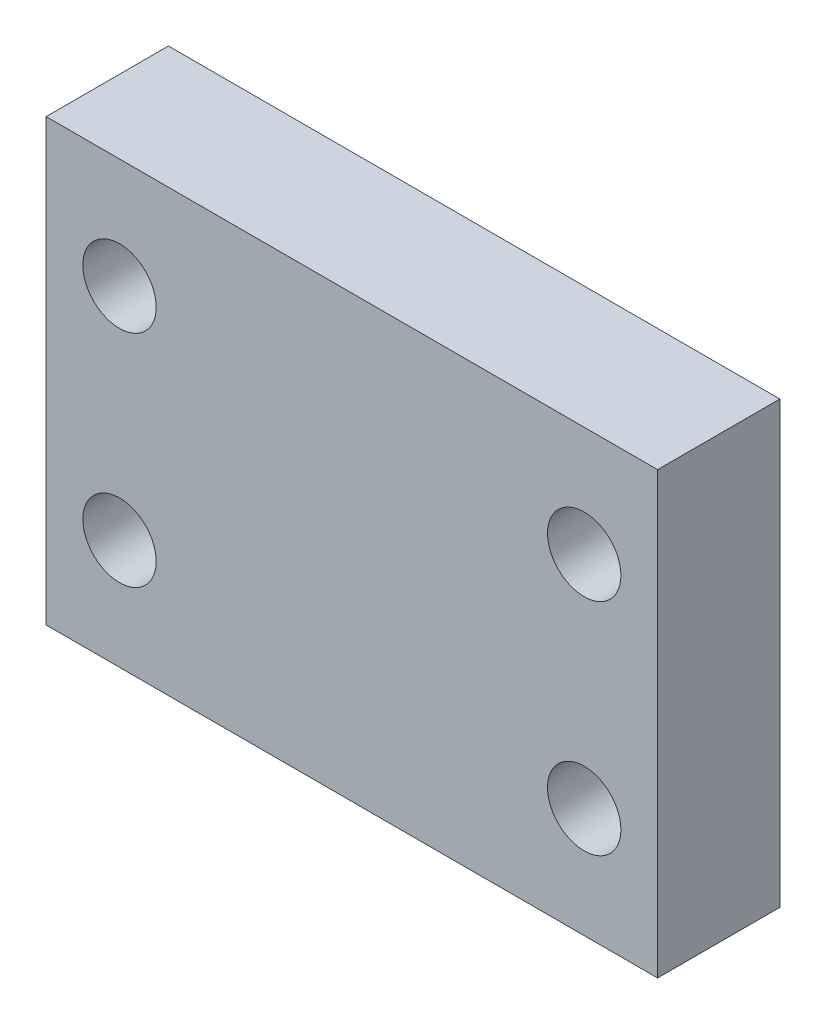
from build123d import *

# Parameters (mm, degrees)
SKETCH1_W           = 25
SKETCH1_H           = 18
SKETCH1_R           = 1.5
BOSS_EXTRUDE1_DEPTH = 5


with BuildPart() as part:
    # Sketch1 → Boss-Extrude1 (new body)
    with BuildSketch(Plane.XY):
        Rectangle(SKETCH1_W, SKETCH1_H)
        with Locations((-9.5, 4.5)):
            Circle(SKETCH1_R, mode=Mode.SUBTRACT)
        with Locations((9.5, 4.5)):
            Circle(SKETCH1_R, mode=Mode.SUBTRACT)
        with Locations((9.5, -4.5)):
            Circle(SKETCH1_R, mode=Mode.SUBTRACT)
        with Locations((-9.5, -4.5)):
            Circle(SKETCH1_R, mode=Mode.SUBTRACT)
    extrude(amount=BOSS_EXTRUDE1_DEPTH)


solid = part.part
